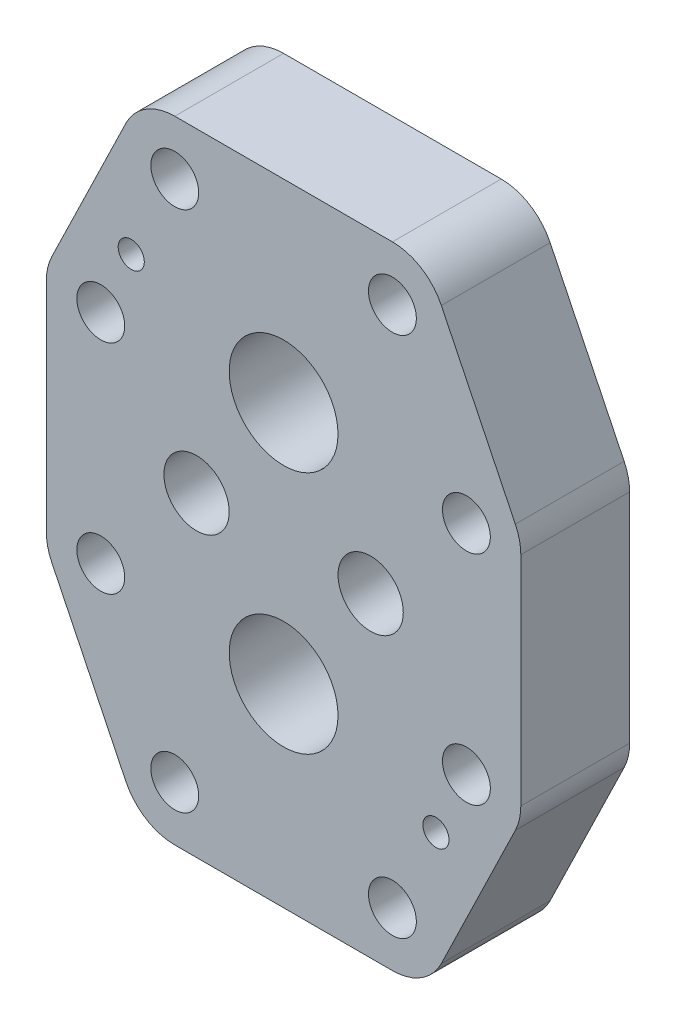
from build123d import *

# Parameters (mm, degrees)
BOSS_EXTRUDE2_DEPTH = 25
SKETCH_19_5_R       = 5.5
SKETCH_19_5_R_2     = 12.5
SKETCH_19_5_R_3     = 7.5
CUT_EXTRUDE1_DEPTH  = 95.082410683
SKETCH_19_6_R       = 3
CUT_EXTRUDE5_DEPTH  = 95.082410683
SKETCH_19_7_2_R     = 4
CUT_EXTRUDE7_DEPTH  = 12


with BuildPart() as part:
    # Sketch 19_7 → Boss-Extrude2 (new body)
    with BuildSketch(Plane.XY):
        with BuildLine():
            Line((54.5, -25), (54.5, 25))
            ThreePointArc((54.5, 25), (54.181915896, 27.801950234), (53.243851982, 30.461299534))
            Line((53.243851982, 30.461299534), (36.243851982, 65.461299534))
            ThreePointArc((36.243851982, 65.461299534), (31.632637327, 70.595193348), (25, 72.5))
            Line((25, 72.5), (-25, 72.5))
            ThreePointArc((-25, 72.5), (-31.632637327, 70.595193348), (-36.243851982, 65.461299534))
            Line((-36.243851982, 65.461299534), (-53.243851982, 30.461299534))
            ThreePointArc((-53.243851982, 30.461299534), (-54.181915896, 27.801950234), (-54.5, 25))
            Line((-54.5, 25), (-54.5, -25))
            ThreePointArc((-54.5, -25), (-54.181915896, -27.801950234), (-53.243851982, -30.461299534))
            Line((-53.243851982, -30.461299534), (-36.243851982, -65.461299534))
            ThreePointArc((-36.243851982, -65.461299534), (-31.632637327, -70.595193348), (-25, -72.5))
            Line((-25, -72.5), (25, -72.5))
            ThreePointArc((25, -72.5), (31.632637327, -70.595193348), (36.243851982, -65.461299534))
            Line((36.243851982, -65.461299534), (53.243851982, -30.461299534))
            ThreePointArc((53.243851982, -30.461299534), (54.181915896, -27.801950234), (54.5, -25))
        make_face()
    extrude(amount=BOSS_EXTRUDE2_DEPTH)

    # 草图19<5> → Cut-Extrude1 (cut, through all)
    with BuildSketch(Plane.XY):
        with Locations((-25, 60)):
            Circle(SKETCH_19_5_R)
        with Locations((-42, 25)):
            Circle(SKETCH_19_5_R)
        with Locations((-42, -25)):
            Circle(SKETCH_19_5_R)
        with Locations((0, -28)):
            Circle(SKETCH_19_5_R_2)
        with Locations((20, 0)):
            Circle(SKETCH_19_5_R_3)
        with Locations((-20, 0)):
            Circle(SKETCH_19_5_R_3)
        with Locations((0, 28)):
            Circle(SKETCH_19_5_R_2)
        with Locations((-25, -60)):
            Circle(SKETCH_19_5_R)
    cut_extrude1 = extrude(amount=CUT_EXTRUDE1_DEPTH, mode=Mode.SUBTRACT)

    # Mirror1: Cut-Extrude1 across plane
    add(cut_extrude1.mirror(Plane(origin=(0, 0, 0), x_dir=(0, 0, 1), z_dir=(1, 0, 0))), mode=Mode.SUBTRACT)

    # 草图19<6> → Cut-Extrude5 (cut, through all)
    with BuildSketch(Plane.XY):
        with Locations((35, -40)):
            Circle(SKETCH_19_6_R)
        with Locations((-35, 40)):
            Circle(SKETCH_19_6_R)
    extrude(amount=CUT_EXTRUDE5_DEPTH, mode=Mode.SUBTRACT)

    # Sketch 19_7 2 → Cut-Extrude7 (cut)
    with BuildSketch(Plane.XY):
        with Locations((-35, 40)):
            Circle(SKETCH_19_7_2_R)
        with Locations((35, -40)):
            Circle(SKETCH_19_7_2_R)
    extrude(amount=CUT_EXTRUDE7_DEPTH, mode=Mode.SUBTRACT)


solid = part.part
